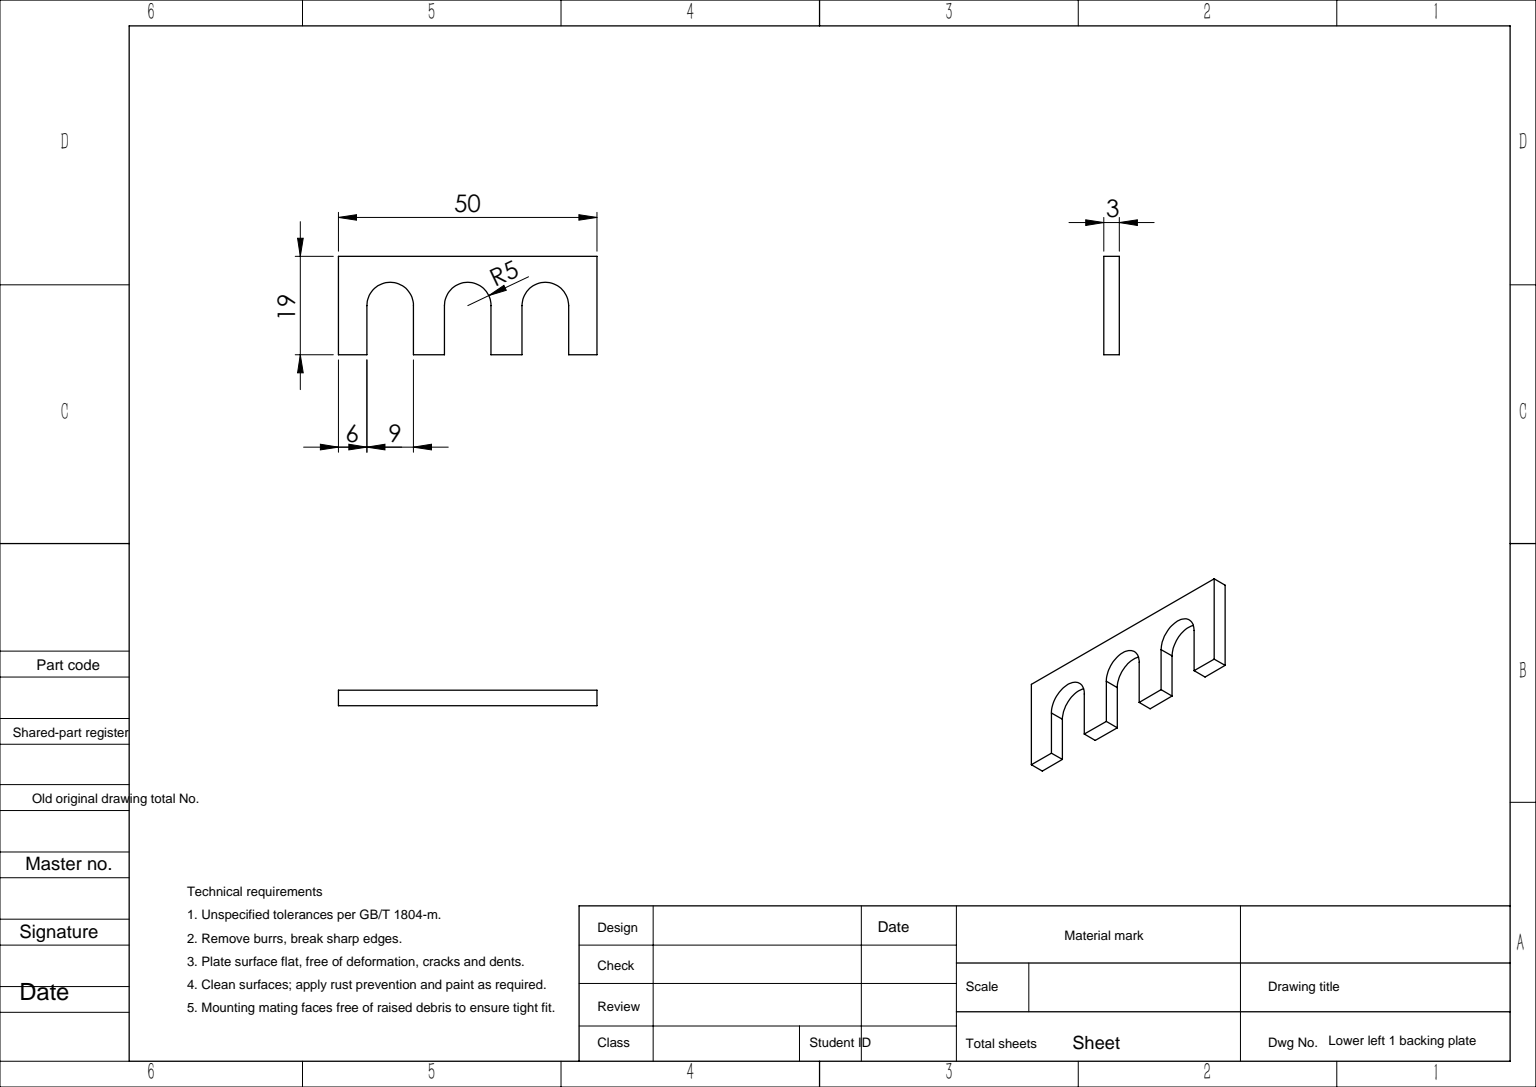
SolidWorks part; units mm, degrees
material "AISI 1045 钢，冷拔"
ref_plane "Front Plane" through (0, 0, 0) normal (0, 0, 1) x (1, 0, 0)
ref_plane "Top Plane" through (0, 0, 0) normal (0, 1, 0) x (1, 0, 0)
ref_plane "Right Plane" through (0, 0, 0) normal (1, 0, 0) x (0, 0, -1)
sketch "Sketch1" plane through (0, 0, 0) normal (0, 0, 1) x (1, 0, 0)
  line L0 (-3.677, 9.5) -> (54.315, 9.5) construction
  line L1 (0, 0) -> (5.5, 0)
  line L2 (0, 0) -> (0, 19)
  line L3 (0, 19) -> (50, 19)
  line L4 (50, 0) -> (50, 19)
  line L5 (5.5, 9.5) -> (5.5, 0)
  line L6 (29.5, 0) -> (35.5, 0)
  line L7 (14.5, 0) -> (14.5, 9.5)
  line L8 (20.5, 9.5) -> (20.5, 0)
  line L9 (29.5, 9.5) -> (29.5, 0)
  line L10 (35.5, 9.5) -> (35.5, 0)
  line L11 (44.5, 9.5) -> (44.5, 0)
  line L12 (14.5, 0) -> (20.5, 0)
  line L13 (44.5, 0) -> (50, 0)
  arc A0 (14.5, 9.5) -> (5.5, 9.5) centre (10, 9.5) ccw
  arc A1 (29.5, 9.5) -> (20.5, 9.5) centre (25, 9.5) ccw
  arc A2 (44.5, 9.5) -> (35.5, 9.5) centre (40, 9.5) ccw
  dimension "D4" = 9
  dimension "D5" = 9
  dimension "D6" = 9
  dimension "D8" = 15
  dimension "D9" = 15
  dimension "D1" = 19
  dimension "D2" = 50
  dimension "D3" = 9.5
  dimension "D7" = 10
extrude "Boss-Extrude1" add sketch "Sketch1" along normal blind 3
